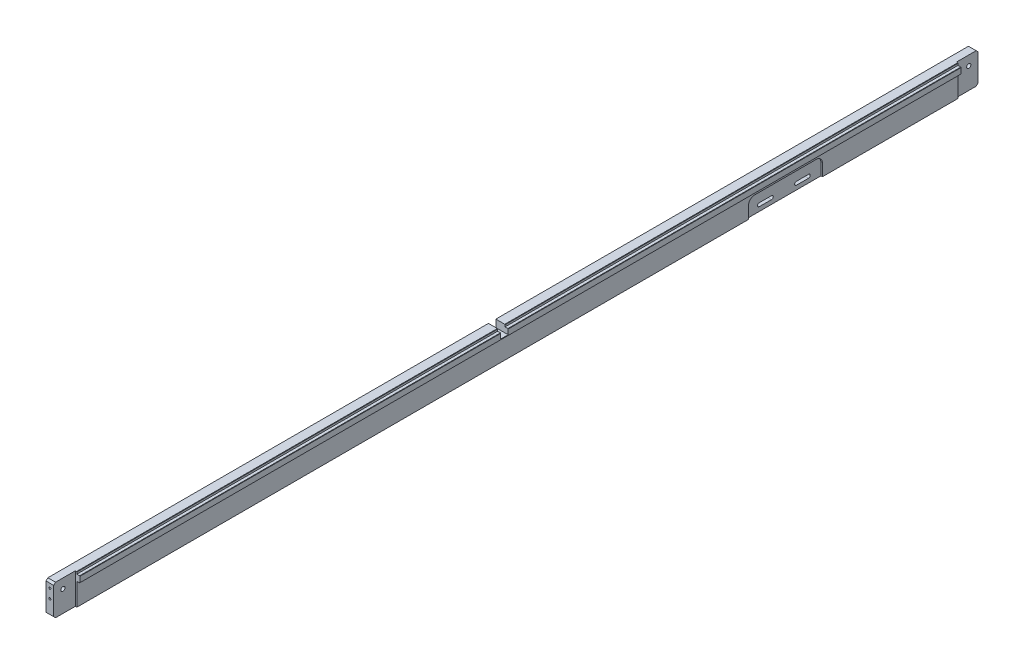
from build123d import *

# Parameters (mm, degrees)
SKETCH_1_W             = 1430
SKETCH_1_H             = 50
EXTRUDE_1_DEPTH        = 15
SKETCH_5_W             = 1430
SKETCH_5_H             = 10
EXTRUDE_3_DEPTH        = 5
HOLE_WIZARD_M6_1_D     = 5
HOLE_WIZARD_M6_1_DEPTH = 17
HOLE_WIZARD_M6_1_TIP   = 1.502151548
CHAMFER_3_SIZE         = 0.5
SKETCH_11_W            = 35
SKETCH_11_H            = 50
EXTRUDE_4_DEPTH        = 12.5
HOLE_WIZARD_M8_1_D     = 6.8
CHAMFER_4_SIZE         = 3
SKETCH_14_W            = 120
SKETCH_14_H            = 29.5
CUT_EXTRUDE_1_DEPTH    = 2.5
CUT_EXTRUDE_2_REACH    = 752.683
FILLET_1_R             = 10
SKETCH_16_W            = 25.507597837
SKETCH_16_H            = 12
CUT_EXTRUDE_3_DEPTH    = 12
HOLE_WIZARD_M6_2_D     = 5
HOLE_WIZARD_M6_2_DEPTH = 17
HOLE_WIZARD_M6_2_TIP   = 1.502151548
HOLE_WIZARD_M4_1_D     = 3.3
HOLE_WIZARD_M4_1_DEPTH = 12
HOLE_WIZARD_M4_1_TIP   = 0.991420021
HOLE_WIZARD_M6_3_D     = 5
HOLE_WIZARD_M6_3_DEPTH = 17
HOLE_WIZARD_M6_3_TIP   = 1.502151548
HOLE_WIZARD_M4_2_D     = 3.3
HOLE_WIZARD_M4_2_DEPTH = 11.5
HOLE_WIZARD_M4_2_TIP   = 0.991420021
HOLE_WIZARD_M4_3_D     = 3.3
HOLE_WIZARD_M4_3_DEPTH = 11.5
HOLE_WIZARD_M4_3_TIP   = 0.991420021


with BuildPart() as part:
    # 草图1 → 凸台-拉伸1 (new body)
    with BuildSketch(Plane(origin=(0, 0, 0), x_dir=(0, 0, -1), z_dir=(1, 0, 0))):
        Rectangle(SKETCH_1_W, SKETCH_1_H)
    extrude(amount=EXTRUDE_1_DEPTH)

    # 草图5 → 凸台-拉伸3 (add)
    with BuildSketch(Plane(origin=(15, 0, 0), x_dir=(0, 0, -1), z_dir=(1, 0, 0))):
        with Locations((0, 16.5)):
            Rectangle(SKETCH_5_W, SKETCH_5_H)
    extrude(amount=EXTRUDE_3_DEPTH)

    # M6 螺纹孔1
    with Locations(Plane(origin=(-8.30723521, -25, 23.598187195), x_dir=(0, 0, -1), z_dir=(0, -1, 0))):
        with Locations((638.598187195, 15.80723521), (593.598187195, 15.80723521), (-266.401812805, 15.80723521), (-221.401812805, 15.80723521)):
            Hole(HOLE_WIZARD_M6_1_D / 2, depth=HOLE_WIZARD_M6_1_DEPTH)
            with Locations((0, 0, -(HOLE_WIZARD_M6_1_DEPTH + HOLE_WIZARD_M6_1_TIP / 2))):  # 118° drill point
                Cone(0, HOLE_WIZARD_M6_1_D / 2, HOLE_WIZARD_M6_1_TIP, mode=Mode.SUBTRACT)

    # 倒角3
    chamfer_3_edges = [part.edges().sort_by_distance(p)[0] for p in [
        (15, 25, 0),
        (20, 21.5, 0),
        (20, 11.5, 0),
    ]]
    chamfer(chamfer_3_edges, length=CHAMFER_3_SIZE)

    # 草图11 → 凸台-拉伸4 (add)
    with BuildSketch(Plane.ZY):
        with Locations((-732.5, 0)):
            Rectangle(SKETCH_11_W, SKETCH_11_H)
        with Locations((732.5, 0)):
            Rectangle(SKETCH_11_W, SKETCH_11_H)
    extrude(amount=-EXTRUDE_4_DEPTH)

    # M8 螺纹孔1 (through all)
    with Locations(Plane(origin=(12.5, 0, 0), x_dir=(0, 0, -1), z_dir=(1, 0, 0))):
        with Locations((735, 9.5), (-735, 9.5)):
            Hole(HOLE_WIZARD_M8_1_D / 2)

    # 倒角4
    chamfer_4_edges = [part.edges().sort_by_distance(p)[0] for p in [
        (6.25, -25, -750),
        (6.25, 25, -750),
        (6.25, -25, 750),
        (6.25, 25, 750),
    ]]
    chamfer(chamfer_4_edges, length=CHAMFER_4_SIZE)

    # 草图14 → 切除-拉伸1 (cut)
    with BuildSketch(Plane(origin=(15, 0, 0), x_dir=(0, 0, -1), z_dir=(1, 0, 0))):
        with Locations((435, -10.25)):
            Rectangle(SKETCH_14_W, SKETCH_14_H)
    extrude(amount=-CUT_EXTRUDE_1_DEPTH, mode=Mode.SUBTRACT)

    # 草图15 → 切除-拉伸2 (cut, up to next)
    with BuildSketch(Plane.ZY, mode=Mode.PRIVATE) as cut_extrude_2_sk1:
        with BuildLine():
            Line((-415, -12.75), (-395, -12.75))
            ThreePointArc((-395, -12.75), (-392.25, -15.5), (-395, -18.25))
            Line((-395, -18.25), (-415, -18.25))
            ThreePointArc((-415, -18.25), (-417.75, -15.5), (-415, -12.75))
        make_face()
    cut_extrude_2_tool1 = extrude(cut_extrude_2_sk1.sketch, amount=-CUT_EXTRUDE_2_REACH, mode=Mode.PRIVATE) & part.part
    # 草图15 → 切除-拉伸2 (cut, up to next)
    with BuildSketch(Plane.ZY, mode=Mode.PRIVATE) as cut_extrude_2_sk2:
        with BuildLine():
            Line((-455, -18.25), (-475, -18.25))
            ThreePointArc((-475, -18.25), (-477.75, -15.5), (-475, -12.75))
            Line((-475, -12.75), (-455, -12.75))
            ThreePointArc((-455, -12.75), (-452.25, -15.5), (-455, -18.25))
        make_face()
    cut_extrude_2_tool2 = extrude(cut_extrude_2_sk2.sketch, amount=-CUT_EXTRUDE_2_REACH, mode=Mode.PRIVATE) & part.part
    add(cut_extrude_2_tool1.solids().sort_by_distance((0, -15.5, -405))[0], mode=Mode.SUBTRACT)
    add(cut_extrude_2_tool2.solids().sort_by_distance((0, -15.5, -465))[0], mode=Mode.SUBTRACT)

    # 圆角1
    fillet_1_edges = [part.edges().sort_by_distance(p)[0] for p in [
        (13.75, 4.5, -375),
        (13.75, 4.5, -495),
    ]]
    fillet(fillet_1_edges, radius=FILLET_1_R)

    # 草图16 → 切除-拉伸3 (cut)
    with BuildSketch(Plane(origin=(0, 25, 0), x_dir=(1, 0, 0), z_dir=(0, 1, 0))):
        with Locations((12.753798919, -26.012)):
            Rectangle(SKETCH_16_W, SKETCH_16_H)
    extrude(amount=-CUT_EXTRUDE_3_DEPTH, mode=Mode.SUBTRACT)

    # M6 螺纹孔2
    with Locations(Plane(origin=(0, -25, 0), x_dir=(-1, 0, 0), z_dir=(0, -1, 0))):
        with Locations((-7.5, -133.513), (-7.5, -158.513)):
            Hole(HOLE_WIZARD_M6_2_D / 2, depth=HOLE_WIZARD_M6_2_DEPTH)
            with Locations((0, 0, -(HOLE_WIZARD_M6_2_DEPTH + HOLE_WIZARD_M6_2_TIP / 2))):  # 118° drill point
                Cone(0, HOLE_WIZARD_M6_2_D / 2, HOLE_WIZARD_M6_2_TIP, mode=Mode.SUBTRACT)

    # M4 螺纹孔1
    with Locations(Plane.ZY):
        with Locations((12.012, 21), (12.012, 9), (40.012, 21), (40.012, 9)):
            Hole(HOLE_WIZARD_M4_1_D / 2, depth=HOLE_WIZARD_M4_1_DEPTH)
            with Locations((0, 0, -(HOLE_WIZARD_M4_1_DEPTH + HOLE_WIZARD_M4_1_TIP / 2))):  # 118° drill point
                Cone(0, HOLE_WIZARD_M4_1_D / 2, HOLE_WIZARD_M4_1_TIP, mode=Mode.SUBTRACT)

    # M6 螺纹孔3
    with Locations(Plane(origin=(0, -25, 0), x_dir=(-1, 0, 0), z_dir=(0, -1, 0))):
        with Locations((-6.25, 287.5), (-6.25, 492.5)):
            Hole(HOLE_WIZARD_M6_3_D / 2, depth=HOLE_WIZARD_M6_3_DEPTH)
            with Locations((0, 0, -(HOLE_WIZARD_M6_3_DEPTH + HOLE_WIZARD_M6_3_TIP / 2))):  # 118° drill point
                Cone(0, HOLE_WIZARD_M6_3_D / 2, HOLE_WIZARD_M6_3_TIP, mode=Mode.SUBTRACT)

    # M4 螺纹孔2
    with Locations(Plane.XY.offset(750)):
        with Locations((6.25, 15), (6.25, 0)):
            Hole(HOLE_WIZARD_M4_2_D / 2, depth=HOLE_WIZARD_M4_2_DEPTH)
            with Locations((0, 0, -(HOLE_WIZARD_M4_2_DEPTH + HOLE_WIZARD_M4_2_TIP / 2))):  # 118° drill point
                Cone(0, HOLE_WIZARD_M4_2_D / 2, HOLE_WIZARD_M4_2_TIP, mode=Mode.SUBTRACT)

    # M4 螺纹孔3
    with Locations(Plane(origin=(0, -25, 0), x_dir=(-1, 0, 0), z_dir=(0, -1, 0))):
        with Locations((-7.5, -42.012), (-7.5, -62.012), (-7.5, -82.012), (-7.5, -102.012), (-7.5, -122.012)):
            Hole(HOLE_WIZARD_M4_3_D / 2, depth=HOLE_WIZARD_M4_3_DEPTH)
            with Locations((0, 0, -(HOLE_WIZARD_M4_3_DEPTH + HOLE_WIZARD_M4_3_TIP / 2))):  # 118° drill point
                Cone(0, HOLE_WIZARD_M4_3_D / 2, HOLE_WIZARD_M4_3_TIP, mode=Mode.SUBTRACT)


solid = part.part
